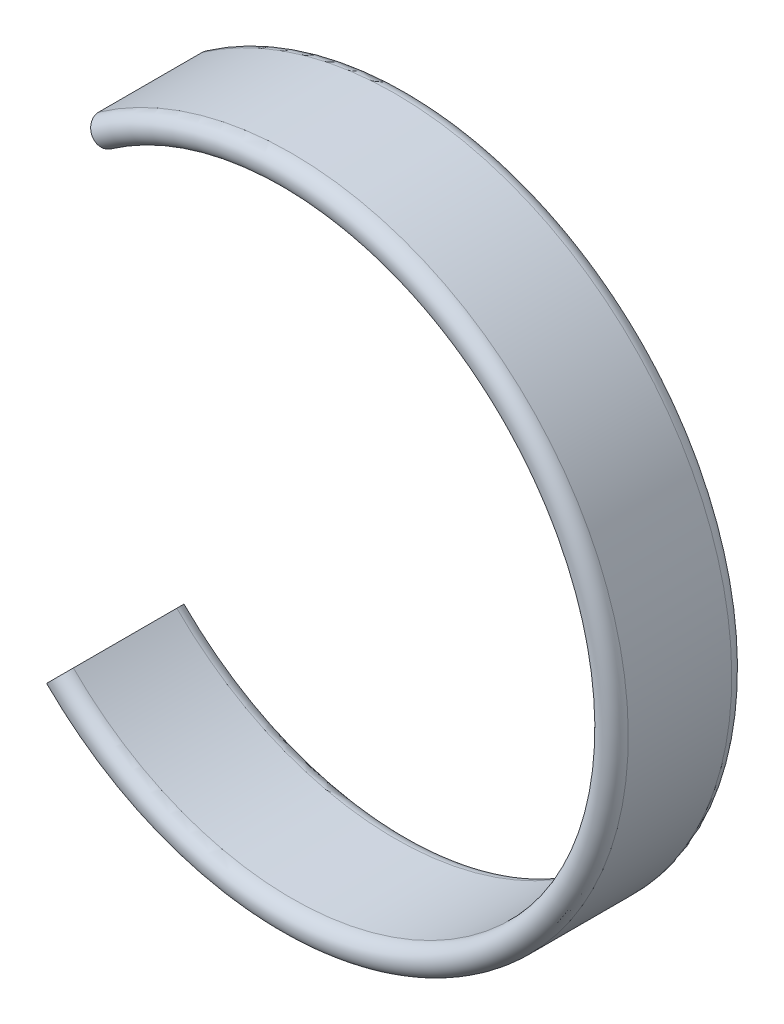
from build123d import *


with BuildPart() as part:
    # Sweep 2: sweep along a path in Sketch 1
    with BuildLine(Plane.XY) as sweep_2_path:
        ThreePointArc((-37.052395334, -37.052395334), (52.20060218, -4.56696092), (-30.055405265, 42.923567121))
    # Sketch 2 → Sweep 2 (sweep)
    with BuildSketch(Plane(origin=(0, 0, 0), x_dir=(-0.5735764363510427, 0.8191520442889942, 0), z_dir=(0.8191520442889942, 0.5735764363510427, 0))):
        with BuildLine():
            Line((50.15, -8.4), (50.15, 8.4))
            ThreePointArc((50.15, 8.4), (52.4, 10.65), (54.65, 8.4))
            Line((54.65, 8.4), (54.65, -8.4))
            ThreePointArc((54.65, -8.4), (52.4, -10.65), (50.15, -8.4))
        make_face()
        with BuildLine():
            Line((50.45, -8.4), (50.45, 8.4))
            ThreePointArc((50.45, 8.4), (52.4, 10.35), (54.35, 8.4))
            Line((54.35, 8.4), (54.35, -8.4))
            ThreePointArc((54.35, -8.4), (52.4, -10.35), (50.45, -8.4))
        make_face(mode=Mode.SUBTRACT)
    sweep(path=sweep_2_path.line)


solid = part.part
